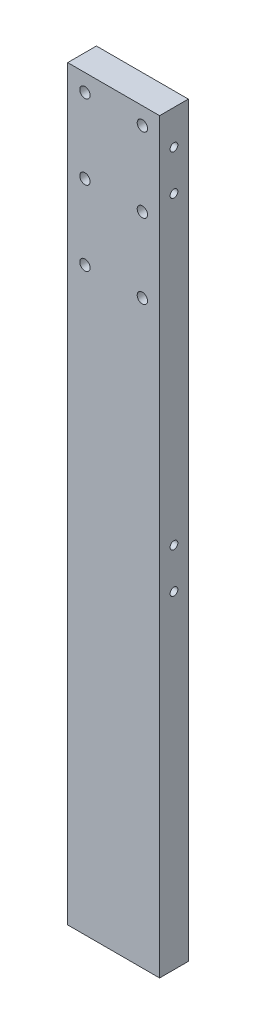
from build123d import *

# Parameters (mm, degrees)
BOSS_EXTRUDE1_DEPTH        = 25
F_9_0_9_DIAMETER_HOLE1_D   = 9
M8_TAPPED_HOLE1_AT_2_COUNT = 2
M8_TAPPED_HOLE1_AT_2_PITCH = 35
LPATTERN1_COUNT            = 2
LPATTERN1_PITCH            = 300


with BuildPart() as part:
    # Sketch1 → Boss-Extrude1 (new body)
    with BuildSketch(Plane.XY):
        Polygon((80, 0), (80, 80), (80, 650), (0, 650), (0, 0), align=None)
    extrude(amount=BOSS_EXTRUDE1_DEPTH)

    # Ø9.0 (9) Diameter Hole1 (through all)
    with Locations(Plane(origin=(15, 635, 25), x_dir=(1, 0, 0), z_dir=(0, 0, 1))):
        with Locations((0, 0), (50, 0), (0, -130), (50, -130), (0, -65), (50, -65)):
            Hole(F_9_0_9_DIAMETER_HOLE1_D / 2)

    # Sketch4 → M8 Tapped Hole1 (revolve, cut)
    with BuildSketch(Plane(origin=(80, 620, 12.5), x_dir=(0, 0, -1), z_dir=(0, 1, 0))):
        Polygon((0, 0), (0, 21.792926105), (3.4, 19.75), (3.4, 0), align=None)
    m8_tapped_hole1 = revolve(axis=Axis((86.35, 620, 12.5), (-1, 0, 0)), mode=Mode.SUBTRACT)

    # M8 Tapped Hole1 at 2: M8 Tapped Hole1 ×2
    with Locations(*[(0, -i * M8_TAPPED_HOLE1_AT_2_PITCH, 0) for i in range(1, M8_TAPPED_HOLE1_AT_2_COUNT)]):
        add(m8_tapped_hole1, mode=Mode.SUBTRACT)

    # LPattern1: M8 Tapped Hole1 ×2
    with Locations(*[(0, -i * LPATTERN1_PITCH, 0) for i in range(1, LPATTERN1_COUNT)]):
        add(m8_tapped_hole1, mode=Mode.SUBTRACT)

    # LPattern1 copy 1 sketch → LPattern1 copy 1 (revolve, cut)
    with BuildSketch(Plane(origin=(80, 285, 12.5), x_dir=(0, 0, -1), z_dir=(0, 1, 0))):
        Polygon((0, 0), (0, 21.792926105), (3.4, 19.75), (3.4, 0), align=None)
    revolve(axis=Axis((86.35, 285, 12.5), (-1, 0, 0)), mode=Mode.SUBTRACT)


solid = part.part
